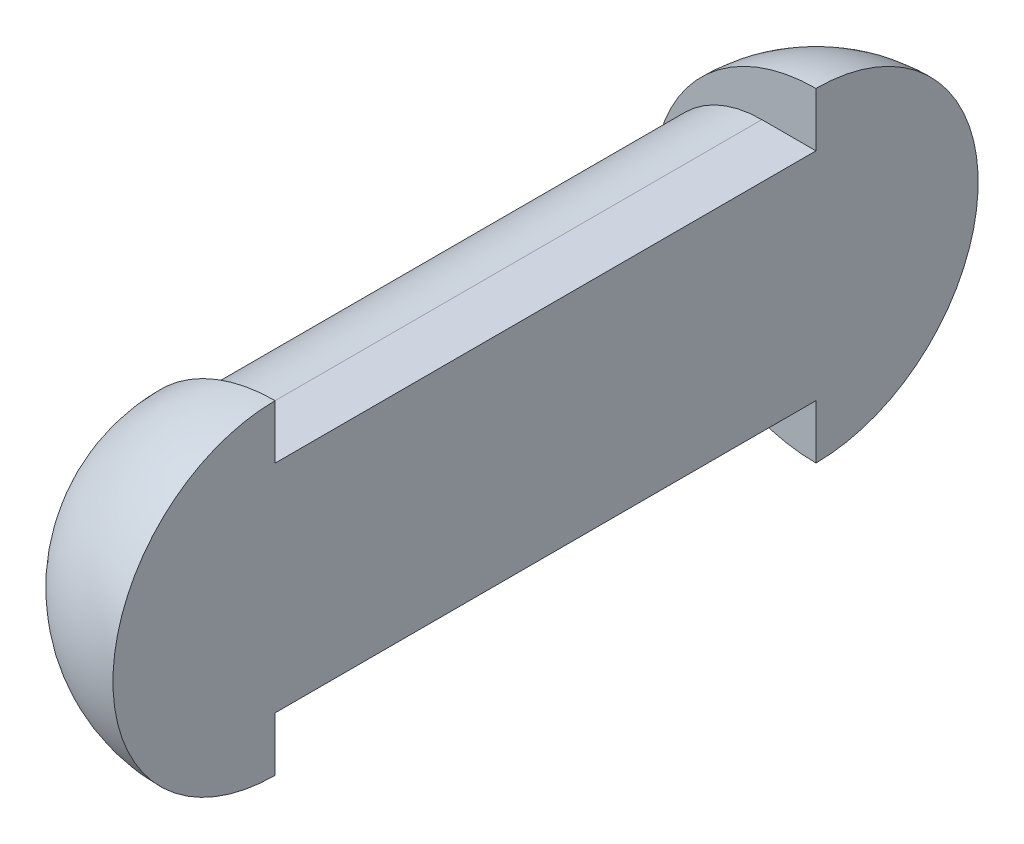
SolidWorks part; units mm, degrees
ref_plane "前视基准面" through (0, 0, 0) normal (0, 0, 1) x (1, 0, 0)
ref_plane "上视基准面" through (0, 0, 0) normal (0, 1, 0) x (1, 0, 0)
ref_plane "右视基准面" through (0, 0, 0) normal (1, 0, 0) x (0, 0, -1)
sketch "草图1" plane through (0, 0, 0) normal (0, 0, 1) x (1, 0, 0)
  line L0 (0, 0) -> (0, -80)
  line L1 (0, -80) -> (-20, -80)
  line L2 (0, 0) -> (-20, 0)
  arc A0 (-20, -80) -> (-20, 0) centre (-20, -40) cw
extrude "凸台-拉伸1" add sketch "草图1" against normal blind 100
sketch3d "3D草图1"
  point P0 (0, -40, -55.8528)
ref_plane "基准面1" through (0, 0, 0) normal (1, 0, 0) x (0, 0, -1)
sketch "草图2" plane through (0, 0, 0) normal (1, 0, 0) x (0, 0, -1)
  line L0 (100, -80) -> (100, 0) construction
  line L1 (100, 20) -> (100, -100)
  arc A0 (100, 20) -> (100, -100) centre (100, -40) cw
revolve "旋转1" add sketch "草图2" angle 90 about L1
mirror "镜向1" about plane through (-20, -40, 0) normal (0, 0, -1) of "旋转1", "凸台-拉伸1"
